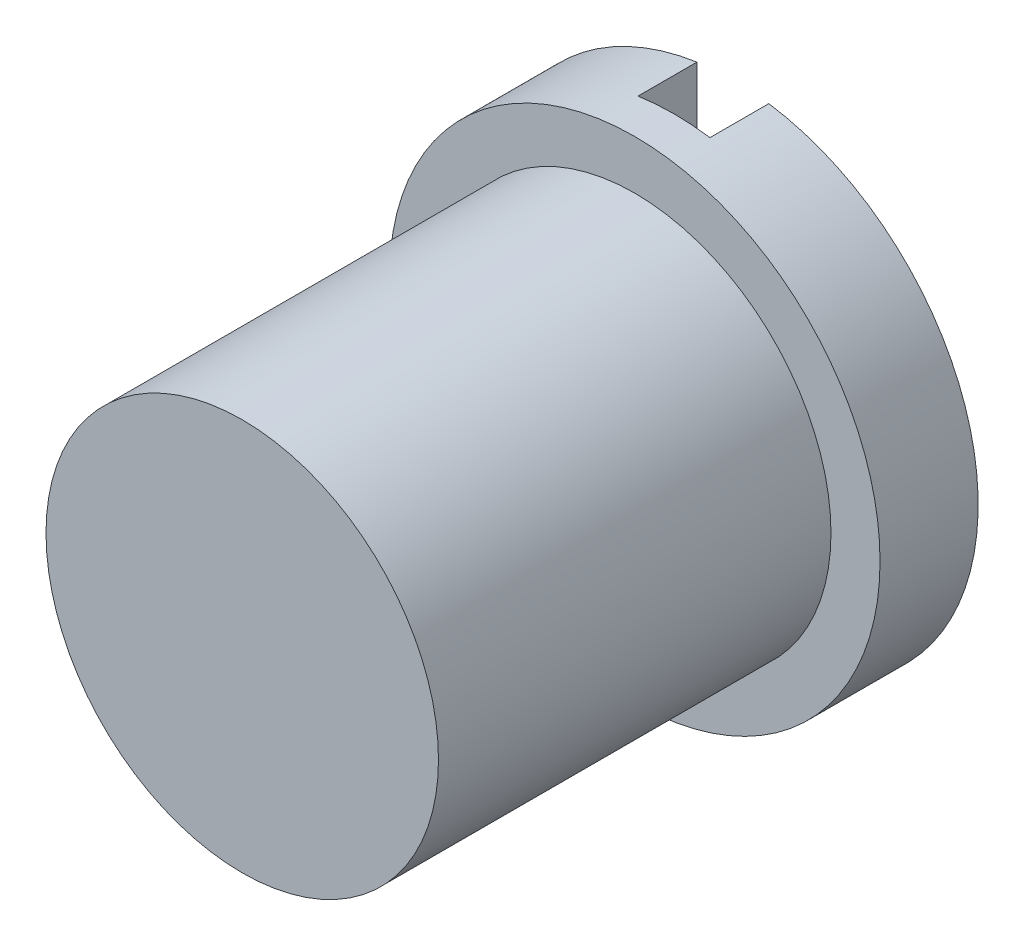
SolidWorks part; units mm, degrees
ref_plane "Front Plane" through (0, 0, 0) normal (0, 0, 1) x (1, 0, 0)
ref_plane "Top Plane" through (0, 0, 0) normal (0, 1, 0) x (1, 0, 0)
ref_plane "Right Plane" through (0, 0, 0) normal (1, 0, 0) x (0, 0, -1)
other "Configuration Table"
sketch "Sketch1" plane through (0, 0, 0) normal (0, 0, 1) x (1, 0, 0)
  circle A0 centre (0, 0) radius 12.5
  dimension "D1" = 25
extrude "Boss-Extrude1" add sketch "Sketch1" along normal blind 5
sketch "Sketch2" plane through (0, 0, 5) normal (0, 0, 1) x (1, 0, 0)
  circle A0 centre (0, 0) radius 10
  dimension "D1" = 20
extrude "Boss-Extrude2" add sketch "Sketch2" along normal blind 20
cosmetic thread "Cosmetic Thread1" parameters "D2"=17.294
sketch "Sketch3" plane through (0, 0, 0) normal (0, 0, -1) x (-1, 0, 0)
  line L0 (0, 12.5) -> (0, -12.5) construction
  line L2 (1.8323, 12.365) -> (1.8323, -12.365)
  line L5 (-1.8323, 12.365) -> (-1.8323, -12.365)
  circle A0 centre (0, 0) radius 12.5 construction
  arc A1 (-1.8323, -12.365) -> (1.8323, -12.365) centre (0, 0) ccw
  arc A2 (1.8323, 12.365) -> (-1.8323, 12.365) centre (0, 0) ccw
extrude "Cut-Extrude2" cut sketch "Sketch3" against normal blind 3
